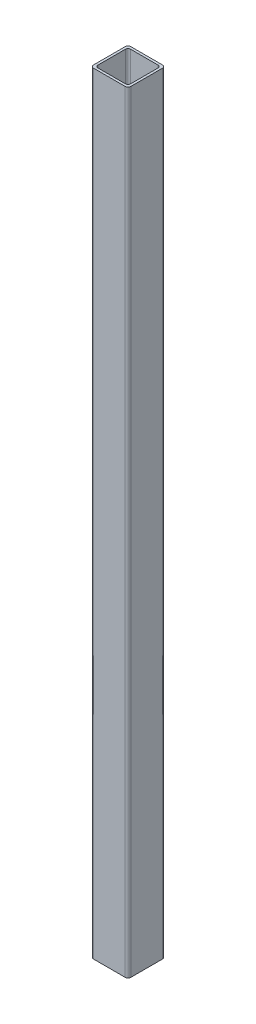
SolidWorks part; units mm, degrees
material "Angle steel 100×100×6/Q235"
ref_plane "Front Plane" through (0, 0, 0) normal (0, 0, 1) x (1, 0, 0)
ref_plane "Top Plane" through (0, 0, 0) normal (0, 1, 0) x (1, 0, 0)
ref_plane "Right Plane" through (0, 0, 0) normal (1, 0, 0) x (0, 0, -1)
sketch "Sketch2" plane through (0, 0, 0) normal (0, 1, 0) x (1, 0, 0)
  line L0 (12.6, 4.775) -> (87.4, 4.775)
  line L1 (6.3, 11.075) -> (6.3, 85.875)
  line L2 (87.4, 92.175) -> (12.6, 92.175)
  line L3 (93.7, 85.875) -> (93.7, 11.075)
  line L4 (7.875, -1.525) -> (92.125, -1.525)
  line L5 (0, 6.35) -> (0, 90.6)
  line L6 (92.125, 98.475) -> (7.875, 98.475)
  line L7 (100, 90.6) -> (100, 6.35)
  arc A0 (100, 90.6) -> (92.125, 98.475) centre (92.125, 90.6) ccw
  arc A1 (92.125, -1.525) -> (100, 6.35) centre (92.125, 6.35) ccw
  arc A2 (0, 6.35) -> (7.875, -1.525) centre (7.875, 6.35) ccw
  arc A3 (7.875, 98.475) -> (0, 90.6) centre (7.875, 90.6) ccw
  arc A4 (12.6, 92.175) -> (6.3, 85.875) centre (12.6, 85.875) ccw
  arc A5 (93.7, 85.875) -> (87.4, 92.175) centre (87.4, 85.875) ccw
  arc A6 (87.4, 4.775) -> (93.7, 11.075) centre (87.4, 11.075) ccw
  arc A7 (6.3, 11.075) -> (12.6, 4.775) centre (12.6, 11.075) ccw
extrude "Boss-Extrude1" add sketch "Sketch2" along normal blind 2070
